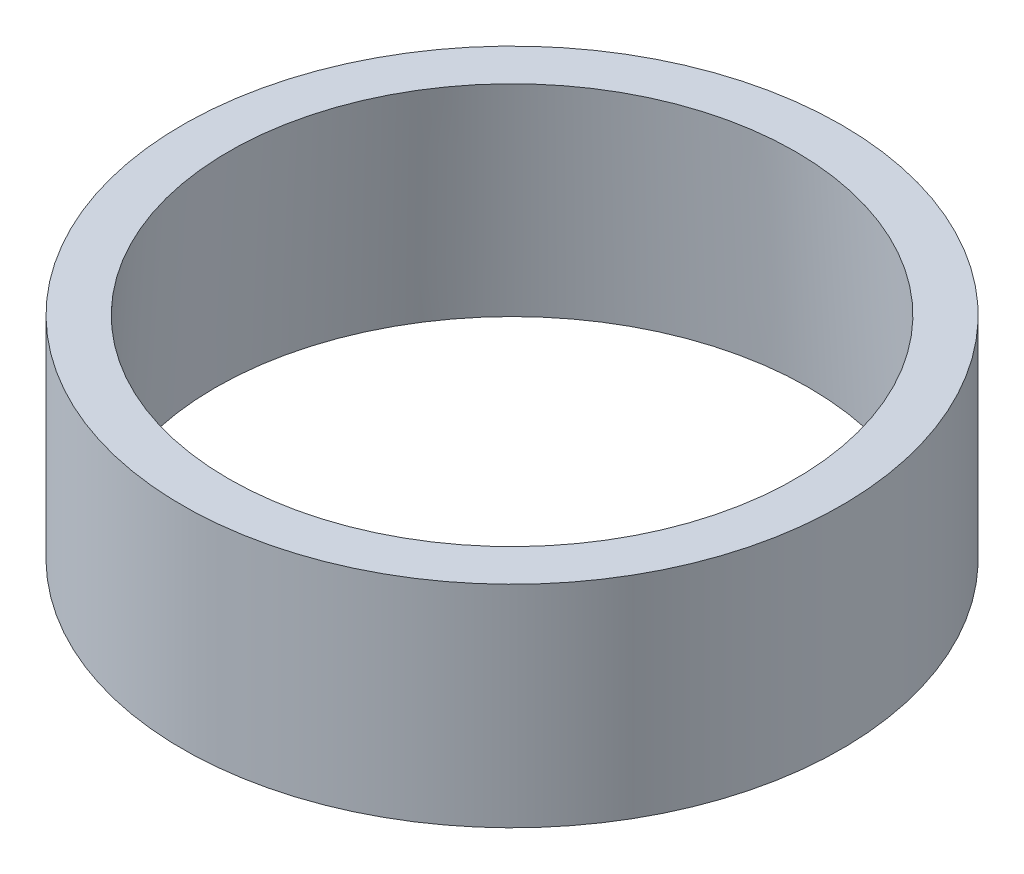
SolidWorks part; units mm, degrees
ref_plane "Front Plane" through (0, 0, 0) normal (0, 0, 1) x (1, 0, 0)
ref_plane "Top Plane" through (0, 0, 0) normal (0, 1, 0) x (1, 0, 0)
ref_plane "Right Plane" through (0, 0, 0) normal (1, 0, 0) x (0, 0, -1)
sketch "Sketch2" plane through (0, 0, 0) normal (0, 0, 1) x (1, 0, 0)
  line L0 (43, 32) -> (45, 0)
  line L1 (45, 0) -> (50, 0)
  line L2 (0, 0) -> (0, 55.7997) construction
  line L3 (43, 32) -> (50, 32)
  line L4 (50, 0) -> (50, 32)
  dimension "D1" = 50
  dimension "D2" = 32
  dimension "D3" = 32
  dimension "D4" = 45
  dimension "D5" = 43
revolve "Revolve1" add sketch "Sketch2" angle 360 about L2
